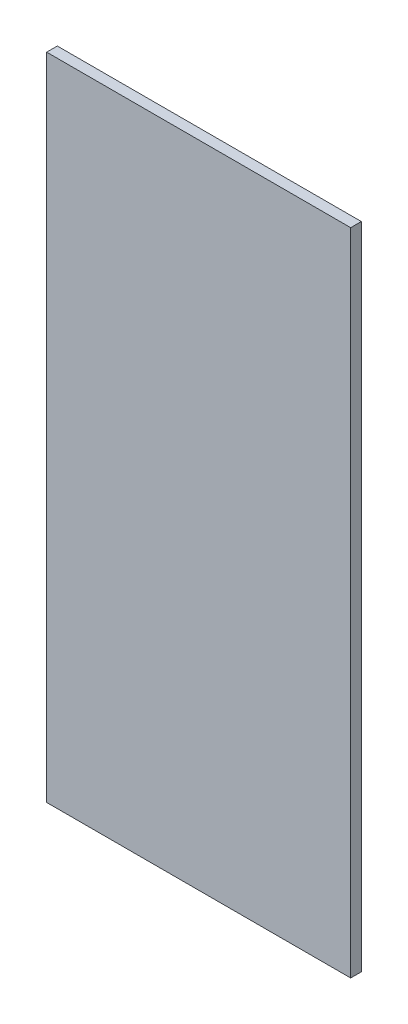
from build123d import *

# Parameters (mm, degrees)
SKETCH1_W           = 400
SKETCH1_H           = 855
BOSS_EXTRUDE1_DEPTH = 7


with BuildPart() as part:
    # Sketch1 → Boss-Extrude1 (new, symmetric)
    with BuildSketch(Plane.XY):
        Rectangle(SKETCH1_W, SKETCH1_H)
    extrude(amount=BOSS_EXTRUDE1_DEPTH, both=True)


solid = part.part
